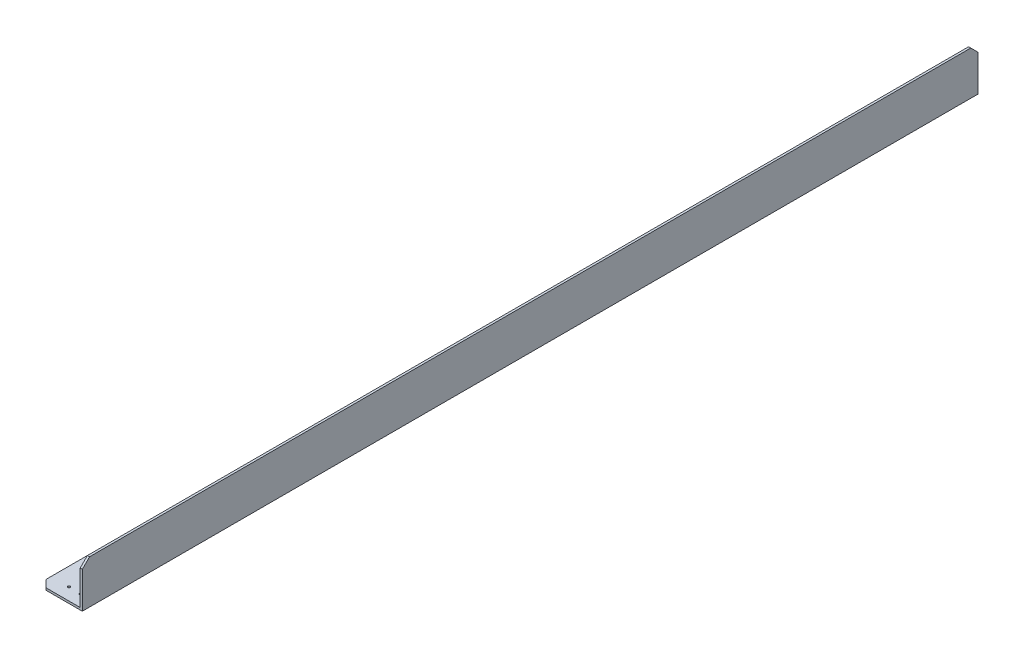
SolidWorks part; units mm, degrees
material "6061Al"
ref_plane "前视基准面" through (0, 0, 0) normal (0, 0, 1) x (1, 0, 0)
ref_plane "上视基准面" through (0, 0, 0) normal (0, 1, 0) x (1, 0, 0)
ref_plane "右视基准面" through (0, 0, 0) normal (1, 0, 0) x (0, 0, -1)
sketch "草图1" plane through (0, 0, 0) normal (0, 0, 1) x (1, 0, 0)
  line L0 (0, 0) -> (60, 0)
  line L1 (60, 0) -> (60, 60)
  line L2 (60, 60) -> (57, 60)
  line L3 (57, 60) -> (57, 3)
  line L4 (57, 3) -> (0, 3)
  line L5 (0, 3) -> (0, 0)
  dimension "D1" = 3
  dimension "D2" = 3
  dimension "D3" = 60
  dimension "D4" = 60
extrude "凸台-拉伸1" add sketch "草图1" along normal mid plane 1234
hole_wizard "M4 螺纹孔2" positions "草图6" profile "草图7" tap size "M4" standard "ISO" end condition up to next
sketch "草图6" plane through (0, 3, 0) normal (0, 1, 0) x (1, 0, 0)
  line L0 (0, 0) -> (153.7715, 0) construction
  point P0 (24.75, 499.9314)
  point P3 (9.75, 484.9314)
  point P6 (39.75, 484.9314)
  point P14 (39.75, -484.9314)
  point P15 (9.75, -484.9314)
  point P16 (24.75, -499.9314)
sketch "草图7" plane through (24.75, 3, -499.9314) normal (1, 0, 0) x (0, 0, 1)
  line L0 (0, 0) -> (0, 3)
  line L1 (0, 3) -> (1.65, 3)
  line L2 (1.65, 3) -> (1.65, 0)
  line L5 (1.65, 0) -> (0, 0)
  line L11 (0, -6.35) -> (0, 107.95) construction
  dimension "通孔螺纹孔钻头直径" = 3.3
  dimension "通孔螺纹孔钻头深度" = 3
cosmetic thread "孔螺蚊线9"
cosmetic thread "孔螺蚊线10"
cosmetic thread "孔螺蚊线11"
cosmetic thread "孔螺蚊线12"
cosmetic thread "孔螺蚊线13"
cosmetic thread "孔螺蚊线14"
hole_wizard "M4 螺纹孔3" positions "草图8" profile "草图9" tap size "M4" standard "ISO" end condition up to next
sketch "草图8" plane through (0, 3, 0) normal (0, 1, 0) x (1, 0, 0)
  line L1 (9.75, 484.9314) -> (39.75, 484.9314) construction
  line L3 (0, 0) -> (109.7061, 0) construction
  line L5 (9.75, -484.9314) -> (39.75, -484.9314) construction
  point P0 (9.75, 484.9314)
  point P3 (39.75, 484.9314)
  point P6 (24.75, 469.9314)
  point P9 (24.75, 499.9314)
  point P23 (24.75, -499.9314)
  point P24 (24.75, -469.9314)
  point P25 (39.75, -484.9314)
  point P26 (9.75, -484.9314)
sketch "草图9" plane through (9.75, 3, -484.9314) normal (1, 0, 0) x (0, 0, 1)
  line L0 (0, 0) -> (0, 3)
  line L1 (0, 3) -> (1.65, 3)
  line L2 (1.65, 3) -> (1.65, 0)
  line L5 (1.65, 0) -> (0, 0)
  line L11 (0, -6.35) -> (0, 107.95) construction
  dimension "通孔螺纹孔钻头直径" = 3.3
  dimension "通孔螺纹孔钻头深度" = 3
cosmetic thread "孔螺蚊线17"
cosmetic thread "孔螺蚊线20"
hole_wizard "M4 间隙孔1" positions "草图10" profile "草图11" hole size "M4" standard "ISO" end condition up to next
sketch "草图10" plane through (0, 3, 0) normal (0, 1, 0) x (1, 0, 0)
  line L0 (0, 0) -> (-189.3751, 0) construction
  line L2 (57, -617) -> (57, 617) construction
  line L3 (42, 0) -> (42, 200) construction
  point P0 (42, 0)
  point P15 (42, 200)
  point P16 (42, 400)
  point P17 (42, 600)
  point P20 (42, -600)
  point P21 (42, -400)
  point P22 (42, -200)
  dimension "D1" = 15
  dimension "D3" = 200
  dimension "D2" = 4
sketch "草图11" plane through (42, 3, 0) normal (1, 0, 0) x (0, 0, 1)
  line L0 (0, 0) -> (0, 3)
  line L1 (0, 3) -> (2.4, 3)
  line L2 (2.4, 3) -> (2.4, 0)
  line L5 (2.4, 0) -> (0, 0)
  line L11 (0, -6.35) -> (0, 107.95) construction
  dimension "通孔孔直径" = 4.8
  dimension "通孔孔深度" = 3
hole_wizard "M4 螺纹孔4" positions "草图12" profile "草图13" tap size "M4" standard "ISO" end condition through all
sketch "草图12" plane through (0, 3, 0) normal (0, 1, 0) x (1, 0, 0)
  line L0 (24.75, 469.9314) -> (24.75, -299.3328) construction
  line L2 (0, 0) -> (161.8694, 0) construction
  line L4 (24.75, 0) -> (24.75, 120) construction
  point P0 (24.75, 0)
  point P19 (24.75, 120)
  point P20 (24.75, 240)
  point P21 (24.75, 360)
  point P22 (24.75, 480)
  point P23 (24.75, 600)
  point P26 (24.75, -600)
  point P27 (24.75, -480)
  point P28 (24.75, -360)
  point P29 (24.75, -240)
  point P30 (24.75, -120)
  dimension "D1" = 6
  dimension "D2" = 120
sketch "草图13" plane through (24.75, 3, 0) normal (1, 0, 0) x (0, 0, 1)
  line L0 (0, 0) -> (0, 3)
  line L1 (0, 3) -> (1.65, 3)
  line L2 (1.65, 3) -> (1.65, 0)
  line L5 (1.65, 0) -> (0, 0)
  line L11 (0, -6.35) -> (0, 107.95) construction
  dimension "通孔螺纹孔钻头直径" = 3.3
  dimension "通孔螺纹孔钻头深度" = 3
cosmetic thread "孔螺蚊线23"
cosmetic thread "孔螺蚊线24"
cosmetic thread "孔螺蚊线25"
cosmetic thread "孔螺蚊线26"
cosmetic thread "孔螺蚊线27"
cosmetic thread "孔螺蚊线28"
cosmetic thread "孔螺蚊线29"
cosmetic thread "孔螺蚊线30"
cosmetic thread "孔螺蚊线31"
cosmetic thread "孔螺蚊线32"
cosmetic thread "孔螺蚊线33"
chamfer "倒角1" distance 10 angle 45 4 edges at (0, 1.5, 617) (58.5, 60, 617) (0, 1.5, -617) (58.5, 60, -617)
